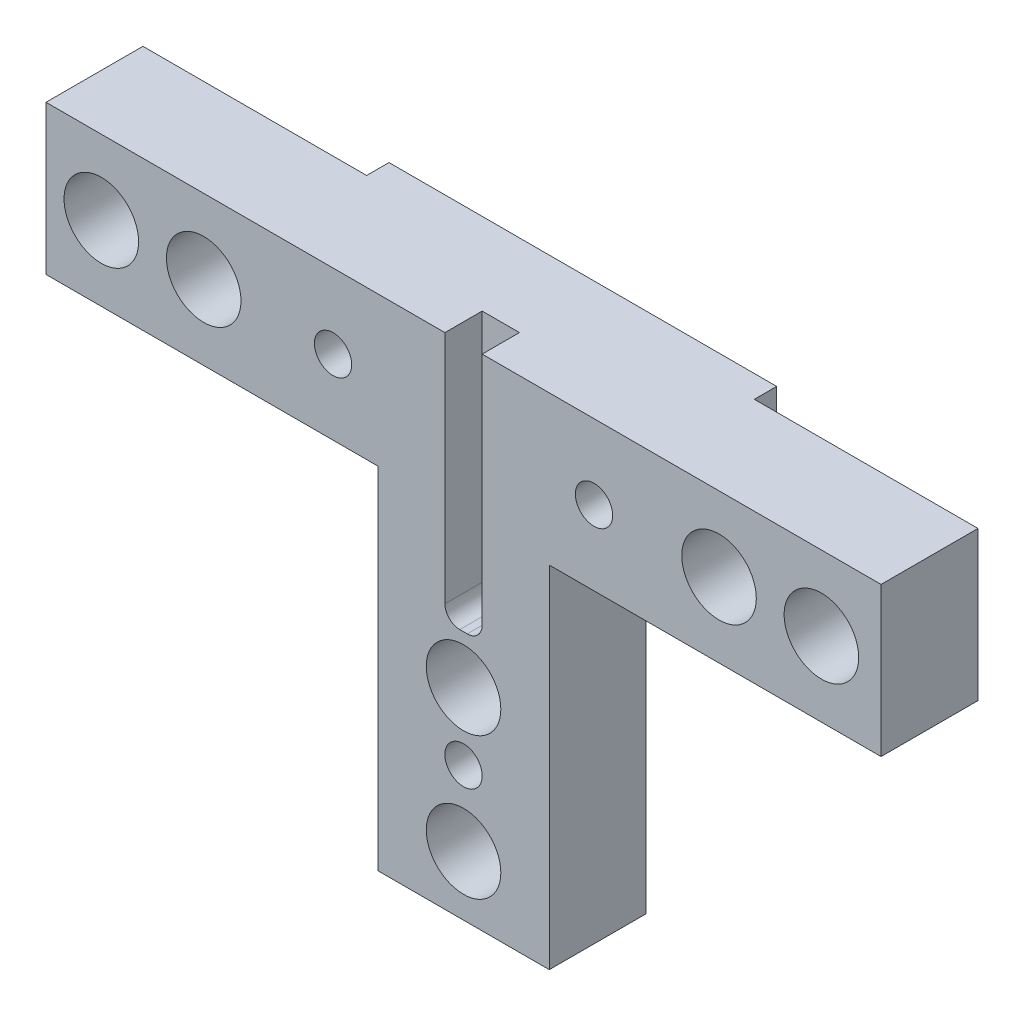
from build123d import *

# Parameters (mm, degrees)
EXTRUDE_1_DEPTH     = 16
SKETCH_2_W          = 30
SKETCH_2_H          = 20
SKETCH_2_W_2        = 23
SKETCH_2_H_2        = 35
CUT_EXTRUDE_1_DEPTH = 3
CUT_EXTRUDE_2_DEPTH = 5
CUT_EXTRUDE_3_REACH = 80.481
SKETCH_4_R          = 2.75
CUT_EXTRUDE_4_REACH = 79.925
SKETCH_5_R          = 2.75
SKETCH_6_R          = 5
CUT_EXTRUDE_5_DEPTH = 9
SKETCH_7_R          = 2.1
CUT_EXTRUDE_6_DEPTH = 12.5
SKETCH_8_R          = 2.5
CUT_EXTRUDE_7_DEPTH = 10


with BuildPart() as part:
    # 草图1 → 凸台-拉伸1 (new body)
    with BuildSketch(Plane.XY):
        Polygon((-47.83180778, 24.741418764), (64.16819222, 24.741418764), (64.16819222, 4.741418764), (19.66819222, 4.741418764), (19.66819222, -42.258581236), (-3.33180778, -42.258581236), (-3.33180778, 4.741418764), (-47.83180778, 4.741418764), align=None)
    extrude(amount=EXTRUDE_1_DEPTH)

    # 草图2 → 切除-拉伸1 (cut)
    with BuildSketch(Plane(origin=(0, 0, 0), x_dir=(-1, 0, 0), z_dir=(0, 0, -1))):
        with Locations((-49.16819222, 14.741418764)):
            Rectangle(SKETCH_2_W, SKETCH_2_H)
        with Locations((-8.16819222, -24.758581236)):
            Rectangle(SKETCH_2_W_2, SKETCH_2_H_2)
        with Locations((32.83180778, 14.741418764)):
            Rectangle(SKETCH_2_W, SKETCH_2_H)
    extrude(amount=-CUT_EXTRUDE_1_DEPTH, mode=Mode.SUBTRACT)

    # 草图3 → 切除-拉伸2 (cut)
    with BuildSketch(Plane.XY.offset(16)):
        with BuildLine():
            Line((10.66819222, 24.741418764), (5.66819222, 24.741418764))
            Line((5.66819222, 24.741418764), (5.66819222, -6.755194133))
            ThreePointArc((5.66819222, -6.755194133), (6.253978657, -8.169407696), (7.66819222, -8.755194133))
            Line((7.66819222, -8.755194133), (8.66819222, -8.755194133))
            ThreePointArc((8.66819222, -8.755194133), (10.082405782, -8.169407696), (10.66819222, -6.755194133))
            Line((10.66819222, -6.755194133), (10.66819222, 24.741418764))
        make_face()
    extrude(amount=-CUT_EXTRUDE_2_DEPTH, mode=Mode.SUBTRACT)

    # 草图4 → 切除-拉伸3 (cut, up to next)
    with BuildSketch(Plane.XY.offset(16), mode=Mode.PRIVATE) as cut_extrude_3_sk1:
        with Locations((56.16819222, 14.741418764)):
            Circle(SKETCH_4_R)
    cut_extrude_3_tool1 = extrude(cut_extrude_3_sk1.sketch, amount=-CUT_EXTRUDE_3_REACH, mode=Mode.PRIVATE) & part.part
    # 草图4 → 切除-拉伸3 (cut, up to next)
    with BuildSketch(Plane.XY.offset(16), mode=Mode.PRIVATE) as cut_extrude_3_sk2:
        with Locations((42.43519222, 14.741418764)):
            Circle(SKETCH_4_R)
    cut_extrude_3_tool2 = extrude(cut_extrude_3_sk2.sketch, amount=-CUT_EXTRUDE_3_REACH, mode=Mode.PRIVATE) & part.part
    # 草图4 → 切除-拉伸3 (cut, up to next)
    with BuildSketch(Plane.XY.offset(16), mode=Mode.PRIVATE) as cut_extrude_3_sk3:
        with Locations((-26.68180778, 14.741418764)):
            Circle(SKETCH_4_R)
    cut_extrude_3_tool3 = extrude(cut_extrude_3_sk3.sketch, amount=-CUT_EXTRUDE_3_REACH, mode=Mode.PRIVATE) & part.part
    # 草图4 → 切除-拉伸3 (cut, up to next)
    with BuildSketch(Plane.XY.offset(16), mode=Mode.PRIVATE) as cut_extrude_3_sk4:
        with Locations((-40.41480778, 14.741418764)):
            Circle(SKETCH_4_R)
    cut_extrude_3_tool4 = extrude(cut_extrude_3_sk4.sketch, amount=-CUT_EXTRUDE_3_REACH, mode=Mode.PRIVATE) & part.part
    add(cut_extrude_3_tool1.solids().sort_by_distance((56.168192, 14.741419, 16))[0], mode=Mode.SUBTRACT)
    add(cut_extrude_3_tool2.solids().sort_by_distance((42.435192, 14.741419, 16))[0], mode=Mode.SUBTRACT)
    add(cut_extrude_3_tool3.solids().sort_by_distance((-26.681808, 14.741419, 16))[0], mode=Mode.SUBTRACT)
    add(cut_extrude_3_tool4.solids().sort_by_distance((-40.414808, 14.741419, 16))[0], mode=Mode.SUBTRACT)

    # 草图5 → 切除-拉伸4 (cut, up to next)
    with BuildSketch(Plane(origin=(0, 0, 3), x_dir=(-1, 0, 0), z_dir=(0, 0, -1)), mode=Mode.PRIVATE) as cut_extrude_4_sk1:
        with Locations((-8.16819222, -15.258581236)):
            Circle(SKETCH_5_R)
    cut_extrude_4_tool1 = extrude(cut_extrude_4_sk1.sketch, amount=-CUT_EXTRUDE_4_REACH, mode=Mode.PRIVATE) & part.part
    # 草图5 → 切除-拉伸4 (cut, up to next)
    with BuildSketch(Plane(origin=(0, 0, 3), x_dir=(-1, 0, 0), z_dir=(0, 0, -1)), mode=Mode.PRIVATE) as cut_extrude_4_sk2:
        with Locations((-8.16819222, -34.258581236)):
            Circle(SKETCH_5_R)
    cut_extrude_4_tool2 = extrude(cut_extrude_4_sk2.sketch, amount=-CUT_EXTRUDE_4_REACH, mode=Mode.PRIVATE) & part.part
    add(cut_extrude_4_tool1.solids().sort_by_distance((8.168192, -15.258581, 3))[0], mode=Mode.SUBTRACT)
    add(cut_extrude_4_tool2.solids().sort_by_distance((8.168192, -34.258581, 3))[0], mode=Mode.SUBTRACT)

    # 草图6 → 切除-拉伸5 (cut)
    with BuildSketch(Plane.XY.offset(16)):
        with Locations((-40.41480778, 14.741418764)):
            Circle(SKETCH_6_R)
        with Locations((-26.68180778, 14.741418764)):
            Circle(SKETCH_6_R)
        with Locations((42.43519222, 14.741418764)):
            Circle(SKETCH_6_R)
        with Locations((56.16819222, 14.741418764)):
            Circle(SKETCH_6_R)
        with Locations((8.16819222, -15.258581236)):
            Circle(SKETCH_6_R)
        with Locations((8.16819222, -34.258581236)):
            Circle(SKETCH_6_R)
    extrude(amount=-CUT_EXTRUDE_5_DEPTH, mode=Mode.SUBTRACT)

    # 草图7 → 切除-拉伸6 (cut)
    with BuildSketch(Plane.XY.offset(16)):
        with Locations((25.66819222, 14.741418764)):
            Circle(SKETCH_7_R)
        with Locations(Location((-9.33180778, 14.741418764, 0), (0, 0, 180))):
            Circle(SKETCH_7_R)
        with Locations((8.16819222, -24.258581236)):
            Circle(SKETCH_7_R)
    extrude(amount=-CUT_EXTRUDE_6_DEPTH, mode=Mode.SUBTRACT)

    # 草图8 → 切除-拉伸7 (cut)
    with BuildSketch(Plane.XY.offset(16)):
        with Locations((-9.33180778, 14.741418764)):
            Circle(SKETCH_8_R)
        with Locations((25.66819222, 14.741418764)):
            Circle(SKETCH_8_R)
        with Locations((8.16819222, -24.258581236)):
            Circle(SKETCH_8_R)
    extrude(amount=-CUT_EXTRUDE_7_DEPTH, mode=Mode.SUBTRACT)


solid = part.part
